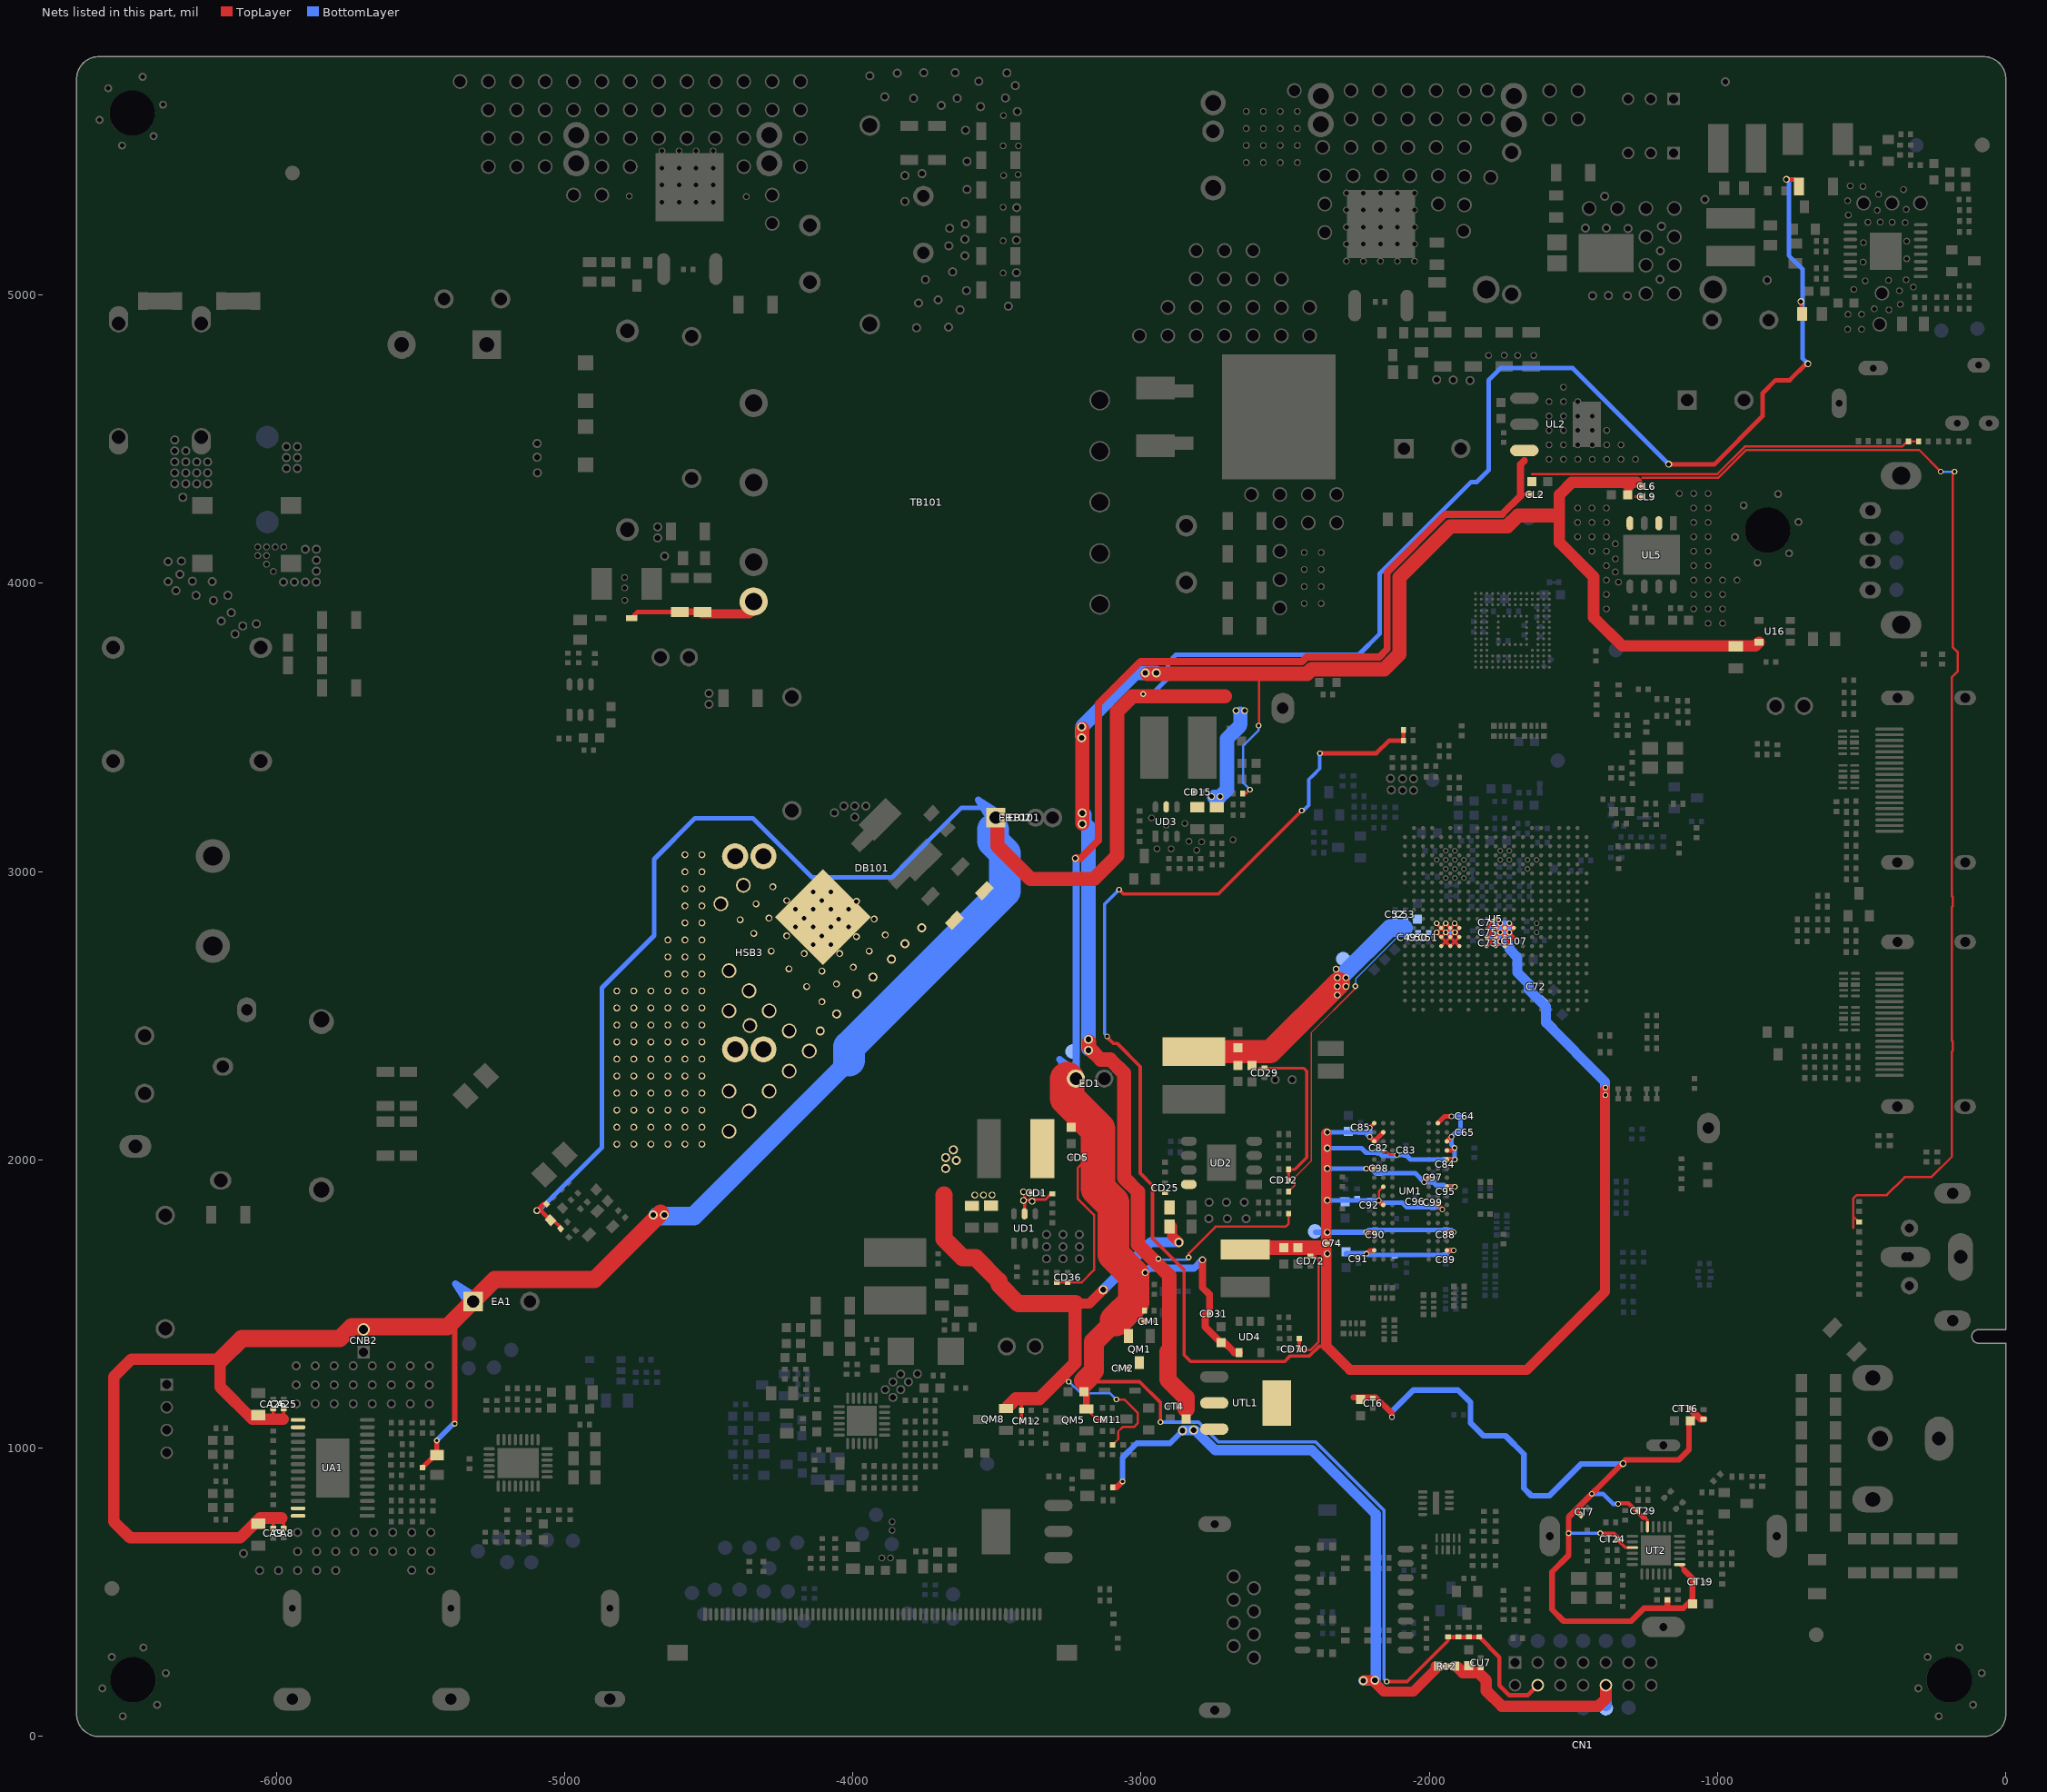
[diagram p0: the nets of this part, all layers, seen from the top]
# Altium PCB MISC84395.PcbDoc (part 9 of 26)
Units mil, origin at the board's own origin, x right, y up, seen from the top; angles counter-clockwise.
Board outline 6692.91 x 5826.77 mil, 2 copper layers (TopLayer, BottomLayer), stack 61.855 mil thick; 951 components, 565 nets, 4374 pads, 1804 vias.
Unrouted connection lines stored in the file: 1.

## Via types
v1: diameter 19.68, hole 11.81, TopLayer to BottomLayer, tented both sides, 1262 vias
v2: diameter 23.62, hole 15.75, TopLayer to BottomLayer, tented both sides, 524 vias
v3: diameter 31.5, hole 19.68, TopLayer to BottomLayer, tented both sides, 11 vias
v4: diameter 24, hole 16, TopLayer to BottomLayer, tented both sides, 6 vias
v5: diameter 19, hole 11.81, TopLayer to BottomLayer, tented both sides, 1 vias

## Nets (pads, with @x,y where several pads share a name; then routed paths per layer and width w, separated by ;. In a path a pad name is that pad's centre, name@x,y a point inside that pad or via, vN(x,y) a via of type N, cw(c..) or ccw(c..) an arc to the next point about the centre after c; other vN are vias at no path point) (continued)
3V3_TUN_IC: CT6.2 CT7.2 CT8.1 CT15.2 CT16.2 CT19.1 CT24.1 CT29.2 CT50.2 LT20.2 RT1.2 UT2.1 UT2.11 UT2.15 UTL1.2 UTL1.4 | length 3570.2
  TopLayer w10: -1334.85,670.48 -1319.68,655.32 UT2.15@-1295.78,655.32 ; -1251,758 -1243.42,750.42 UT2.11@-1243.42,727.36 ; UT2.1@-1117.02,596.26 UT2.1@-1132,596.26 -1116.5,580.76 -1116.5,577.5
  TopLayer w12: v1@-1406.82,704.82 -1358.97,704.82 -1345.48,691.34 -1345.48,680.45 -1335.39,670.35
  TopLayer w15: -1491.7,785.96 CT7.2@-1473.87,768.13 ; v1@-1343,809 -1309.42,809 -1259.97,759.55 -1251,759.55
  TopLayer w20: -2264,1176.11 -2185.43,1176.11 -2130,1120.68 ; -1174.21,447.5 RT1.2@-1174.21,474.46 ; -1116.5,577.5 -1087.44,548.44 -1087.44,476.74 ; CT8.1@-1095.5,468.68 -1118.71,445.47 -1255.17,445.47 -1300.25,400.39 -1534.23,400.39 -1574.5,440.66 -1574.5,571 -1516.97,628.53 v1(-1516.97,705) -1516.97,761.16 -1321.1,957.03 -1318.6,959.53 -1135.31,959.53 -1099.4,995.44 -1099.4,1089.79 -1098.4,1090.79 CT15.2@-1094.19,1095
  TopLayer w24: CT15.2@-1097.19,1096 CT15.2@-1096.26,1096.93 ; CT16.2@-1096.26,1137.27 -1059.26,1100.26 LT20.2@-1049,1100.26
  BottomLayer w12: v1@-1515.91,705 v1@-1408,705
  BottomLayer w15: v1(-1436.29,841.84) -1398.24,841.84 -1363.4,807 v1(-1345,807)
  BottomLayer w20: v1(-2130,1108) -2130,1127.65 -2055.8,1201.84 -1900.35,1201.84 -1857.41,1158.9 -1857.41,1088.41 -1812,1043 -1736,1043 -1672,979 -1672,860.75 -1646.25,835 -1583.89,835 -1473.59,945.3 v2@-1326.3,945.3
  other v1: -1407,705
  other v2: -1328,946.5
5V_M: CL5.2 CL6.2 CL9.2 CM2.1 CT3.2 CT4.1 CU.1 pad.VIA5@-2189,195 pad.VIA5@-2228.87,194.13 pad.VIA5@-2818,1063 pad.VIA5@-2856,1061 pad.VIA5@-2947.23,3688.77 pad.VIA5@-2985.23,3688.77 pad.VIA5@-3182.5,2380 pad.VIA5@-3182.5,2418 pad.VIA5@-3204,3165 pad.VIA5@-3204,3203 pad.VIA5@-3206,3464 pad.VIA5@-3206,3502 QM1.D R12.1 RD25.2 RD26.2 RG02.2 RI1.1 U16.5 UL5.2 UL5.4 UTL1.3 | length 13409.1
  TopLayer w8: v1(-2835,1662) -2835,1675.52 -2741.87,1768.65 -2499.35,1768.65 -2488.27,1779.73 RD25.2@-2488.27,1814 ; RD26.2@-2645.68,3269 RD26.2@-2647.56,3270.87 -2635.13,3270.87 v1(-2622,3284) ; v1@-2590.16,3508.58 -2590.16,3685.84 ; -1261,4366 -997,4366 -900.94,4462.06 -301.06,4462.06 v1(-226,4387) ; -530,1764.47 -530,1866.16 -518,1878.16 -413.16,1878.16 -351.32,1940 -258.85,1940 -187.74,2011.11 -187.74,2376.16 -184.99,2378.91 -184.99,2411.09 -187.74,2413.84 -187.74,2877.16 -184.99,2879.91 -184.99,2912.09 -187.74,2914.84 -187.74,3673.85 -167.5,3694.09 ; -530,1805 RI1.1@-509,1784 ; -184.83,3676.76 -167.5,3694.09 ; v1(-178,4387) -181,4387 -184.83,4383.17 -184.83,3779.24 -167.5,3761.91 -167.5,3694.09
  TopLayer w12: -1284.37,4336 CL6.2@-1263.11,4336 ; -1282.37,4300 CL9.2@-1263.11,4300
  TopLayer w20: RG02.2@-3098.27,864 -3085,864 v1(-3064.5,884.5)
  TopLayer w35: pad.VIA5@-2228,195 -2197.74,195 -2158.74,156 -2055.78,156 -1978.64,233.14 R12.1@-1978.64,244
  TopLayer w40: -1320.21,4350 -1308.2,4338 ; -1280.84,4350 -1506,4350 -1548.83,4307.17 -1548.83,4140.87 -1430.15,4022.18 -1430.15,3881.42 -1331.75,3783.02 -868.54,3783.02 U16.5@-855.97,3795.6
  TopLayer w50: pad.VIA5@-3203.84,3167 pad.VIA5@-3203.84,3495 ; pad.VIA5@-3180,2388 pad.VIA5@-3180,2409 ; pad.VIA5@-3177.25,2385.25 -3140.16,2348.16 -3106.98,2348.16 -3059,2300.18 -3059,1937.44 -3011,1889.44 -3011,1706.64 -2902,1597.64 -2902,1349 ; pad.VIA5@-2978,3686 -2423.73,3686 ; -2407.99,3701.75 -2423.73,3686 ; -1556.84,4235 -1691.9,4235 -1729.9,4197 -1926.83,4197 -2103.88,4019.95 -2103.88,3754.12 -2156,3702 -2407.73,3702 -2423.73,3686
  TopLayer w60: -2907,1334 -2907,1238 -2844,1175 -2844,1136
  BottomLayer w8: v1@-2939.5,1656.5 -2942,1654 -2843,1654 v1(-2835,1662) ; v1(-2622,3284) -2645.27,3307.27 -2645.27,3436.72 -2592.7,3489.29 v1(-2592.7,3506.03) ; v1(-226,4387) v1(-178,4387)
  BottomLayer w20: v1(-3064.5,884.5) -3064.29,884.71 -3064.29,967.68 -3015.16,1016.82 -2900.18,1016.82 pad.VIA5@-2856,1061
  BottomLayer w35: pad.VIA5@-2854,1062 -2812,1062 -2743.5,993.5 -2406.81,993.5 -2186,772.69 -2186,198 -2189.87,194.13 pad.VIA5@-2228.87,194.13
  BottomLayer w50: pad.VIA5@-3204,3469 -3204,3503.57 -3018.8,3688.77 pad.VIA5@-2985.23,3688.77 pad.VIA5@-2947.23,3688.77 ; pad.VIA5@-3197,3197 -3197,3169 -3182.5,3154.5 pad.VIA5@-3182.5,2418 pad.VIA5@-3182.5,2386
  other v1: -2940,1657
5V_STB: 5V_STB.1 CD5.1 CD8.2 CD31.2 CD36.2 CD69.2 CL1.2 CL2.1 CM1.1 CM3.2 CM11.2 CN1.4 ED1.1 LD1.2 QM1.S QM5.S RD1.2 RK3.2 RK5.1 RK6.2 RK12.2 RM1.2 RV15.2 RV17.2 UD4.4 UL2.3 | length 10351.8
  TopLayer w8: RD1.2@-3292,1575.54 -3205.46,1575.54 -3163,1618 -3163,1809 -3220,1866 -3220,1972 -3191,2001 ; QM5.S@-3189.76,1135.4 -3153.35,1099 CM11.2@-3133.73,1099 ; -2116.88,4072 -1975.44,4213.44 ; -1644,4378.5 -1643.5,4379 -1000.83,4379 -905.87,4473.96 -359.9,4473.96 -341.69,4492.16 RV15.2@-338.1,4492.16 -302.73,4492.16 RV17.2@-302.57,4492
  TopLayer w12: -3163.1,1230.66 -3005.44,1230.66 -2932.5,1157.72 v1(-2932.5,1090.5) ; v1(-2148,191) -2077,191 -1935,333 RK6.2@-1935,345.27 ; -1686.34,4316 -1684.33,4318 -1674.34,4308 CL2.1@-1649.73,4308
  TopLayer w15: -3025.92,1477.19 CM1.1@-2988.73,1440 ; RK6.2@-1935,345.27 RK5.1@-1861,345.27 ; RK3.2@-1889.33,345.27 RK5.1@-1861,345.27 ; RK12.2@-1824,345.27 RK12.2@-1827.21,345.27 ; CN1.4@-1624.01,178 -1659.02,143 -1723,143 -1756.91,176.91 -1756.91,274.97 RK12.2@-1827.21,345.27 ; RK5.1@-1861,345.27 RK12.2@-1827.21,345.27
  TopLayer w25: v2(-3228,3046) -3210,3046 ; v2@-3223,3046 -3210,3046 ; QM5.S@-3189.76,1135.4 -3189.76,1204 -3163.1,1230.66 ; v2(-2787.5,1653) -2787.5,1557.74 -2762.66,1532.89 -2762.66,1477.11 -2777.5,1462.26 -2777.5,1420.88 -2724.62,1368 -2712,1368 -2676.15,1332.15 UD4.4@-2659.61,1332.15 ; -2120.43,4063.5 -2146.38,4037.55 ; -1670.54,4425.45 -1684.33,4411.65 -1684.33,4318 -1684.33,4302.67 -1747.5,4239.5 -1944.43,4239.5 -2146.38,4037.55 ; -3210,3046 -3148.34,3107.66 -3148.34,3582 -3001.84,3728.5 -2441.34,3728.5 -2425.34,3744.5 -2173.6,3744.5 -2146.38,3771.72 -2146.38,4037.55
  TopLayer w70: -3198.06,1233.75 -3163.5,1268.31 -3163.5,1368.3 -3088.4,1443.4
  TopLayer w110: -3101,1852.16 -3096,1847.16 -3096,1671.43 -3025.92,1601.35 -3025.92,1505.88 -3088.4,1443.4
  TopLayer w120: ED1.1@-3256.84,2280.07 -3256.84,2213.93 -3149,2106.09 ; -3198,2156 -3149,2107 -3149,2106.09 ; -3101,1852.16 -3149,1900.16 -3149,2106.09
  BottomLayer w12: v1(-2932.5,1090.5) -2800.19,1090.5 -2731.69,1022 -2395,1022 -2157.5,784.5 -2157.5,200.5 v1(-2148,191)
  BottomLayer w25: ED1.1@-3225,2308.51 v2@-3225,3046 ; v2(-2986,1609) -2971,1624 -2816.5,1624 v2(-2787.5,1653)
5V_WIFI: 5V_WIFI.1 CN1.10 CU6.1 CU7.1 R12.2 R12.3 | length 725.1
  TopLayer w15: CN1.10@-1387.8,171.67 CN1.10@-1387.8,178
  TopLayer w40: R12.2@-1902,240 -1884,222 -1830,222 -1803,195 -1803,159 -1749,105 -1414,105 -1387.8,131.2 CN1.10@-1387.8,178
  BottomLayer w40: 5V_WIFI.1@-1387.74,108 CN1.10@-1387.74,177.95
12V: CA1.2 CA2.2 CA8.2 CA9.2 CA25.1 CA26.2 CD1.2 CD4.1 CD6.1 CD13.1 CD14.1 CD15.1 CD23.2 CD24.2 CD25.2 CM12.2 CNB2.2 DB101.2 EA1.1 EB101.1@-3504,3187 EB102.1@-3504,3187 HSB3.1 HSB3.2 HSB3.3 HSB3.4 pad.VIA5@-2641,3558 pad.VIA5@-2671,3558 pad.VIA5@-2726,3260 pad.VIA5@-2756,3260 pad.VIA5@-2869,1714 pad.VIA5@-3131.42,1549.58 pad.VIA5@-3378,1857 pad.VIA5@-3408,1859 pad.VIA5@-3408,1889 pad.VIA5@-3517,1878 pad.VIA5@-3547,1878 pad.VIA5@-3577,1878 pad.VIA5@-3641.13,1998.13 pad.VIA5@-3651,2035 pad.VIA5@-3677.87,1970.13 pad.VIA5@-3677.87,2008.13 pad.VIA5@-3761,2805 pad.VIA5@-3819,2750 pad.VIA5@-3866,2696 pad.VIA5@-3930,2634 pad.VIA5@-3986,2576 pad.VIA5@-4056,2506 pad.VIA5@-4113,2447 pad.VIA5@-4150.99,2377.82 pad.VIA5@-4220.58,2308.22 pad.VIA5@-4220.58,2447.42 pad.VIA5@-4290.18,2238.63 pad.VIA5@-4290.18,2517.02 pad.VIA5@-4357,2466 pad.VIA5@-4359.78,2169.03 pad.VIA5@-4359.78,2586.61 pad.VIA5@-4379.6,2952.4 pad.VIA5@-4429.37,2099.43 pad.VIA5@-4429.37,2238.63 pad.VIA5@-4429.38,2517.02 pad.VIA5@-4429.38,2656.21 pad.VIA5@-4457.6,2888.4 pad.VIA5@-4523.38,2054.38 pad.VIA5@-4523.38,2113.43 pad.VIA5@-4523.38,2172.49 pad.VIA5@-4523.38,2231.54 pad.VIA5@-4523.38,2290.6 pad.VIA5@-4523.38,2349.65 pad.VIA5@-4523.38,2408.71 pad.VIA5@-4523.38,2467.76 pad.VIA5@-4523.38,2526.82 pad.VIA5@-4523.38,2585.87 pad.VIA5@-4523.38,2644.93 pad.VIA5@-4523.38,2703.99 pad.VIA5@-4523.38,2763.04 pad.VIA5@-4523.38,2822.1 pad.VIA5@-4523.38,2881.15 pad.VIA5@-4523.38,2940.21 pad.VIA5@-4523.38,2999.26 pad.VIA5@-4523.38,3058.32 pad.VIA5@-4582.44,2054.38 pad.VIA5@-4582.44,2113.43 pad.VIA5@-4582.44,2172.49 pad.VIA5@-4582.44,2231.54 pad.VIA5@-4582.44,2290.6 pad.VIA5@-4582.44,2349.65 pad.VIA5@-4582.44,2408.71 pad.VIA5@-4582.44,2467.76 pad.VIA5@-4582.44,2526.82 pad.VIA5@-4582.44,2585.87 pad.VIA5@-4582.44,2644.93 pad.VIA5@-4582.44,2703.99 pad.VIA5@-4582.44,2763.04 pad.VIA5@-4582.44,2822.1 pad.VIA5@-4582.44,2881.15 pad.VIA5@-4582.44,2940.21 pad.VIA5@-4582.44,2999.26 pad.VIA5@-4582.44,3058.32 pad.VIA5@-4641.49,2054.38 pad.VIA5@-4641.49,2113.43 pad.VIA5@-4641.49,2172.49 pad.VIA5@-4641.49,2231.54 pad.VIA5@-4641.49,2290.6 pad.VIA5@-4641.49,2349.65 pad.VIA5@-4641.49,2408.71 pad.VIA5@-4641.49,2467.76 pad.VIA5@-4641.49,2526.82 pad.VIA5@-4641.49,2585.87 pad.VIA5@-4641.49,2644.93 pad.VIA5@-4641.49,2703.99 pad.VIA5@-4641.49,2763.04 pad.VIA5@-4654,1809 pad.VIA5@-4692,1809 pad.VIA5@-4700.55,2054.38 pad.VIA5@-4700.55,2113.43 pad.VIA5@-4700.55,2172.49 pad.VIA5@-4700.55,2231.54 pad.VIA5@-4700.55,2290.6 pad.VIA5@-4700.55,2349.65 pad.VIA5@-4700.55,2408.71 pad.VIA5@-4700.55,2467.76 pad.VIA5@-4700.55,2526.82 pad.VIA5@-4700.55,2585.87 pad.VIA5@-4759.6,2054.38 pad.VIA5@-4759.6,2113.43 pad.VIA5@-4759.6,2172.49 pad.VIA5@-4759.6,2231.54 pad.VIA5@-4759.6,2290.6 pad.VIA5@-4759.6,2349.65 pad.VIA5@-4759.6,2408.71 pad.VIA5@-4759.6,2467.76 pad.VIA5@-4759.6,2526.82 pad.VIA5@-4759.6,2585.87 pad.VIA5@-4818.66,2054.38 pad.VIA5@-4818.66,2113.43 pad.VIA5@-4818.66,2172.49 pad.VIA5@-4818.66,2231.54 pad.VIA5@-4818.66,2290.6 pad.VIA5@-4818.66,2349.65 pad.VIA5@-4818.66,2408.71 pad.VIA5@-4818.66,2467.76 pad.VIA5@-4818.66,2526.82 pad.VIA5@-4818.66,2585.87 QM8.S R27.2 RA25.1 RA27.1 RB128.2 RB129.2 RB131.2 RB135.1 RB158.2 RB816.2 RB826.2 RD2.1 RM2.1 UA1.15 UA1.16 UA1.27 UA1.28 UD1.5 UD2.8 UD3.5 | length 17762
  TopLayer w8: -3271.72,1251.72 v1(-3251,1231) ; R27.2@-3099,1011.73 -3079.41,1031.32 -3079.41,1058.09 -3063.75,1073.75 -3024.41,1073.75 -3012,1086.16 -3012,1123 -3058,1169 v1(-3086,1169)
  TopLayer w10: UD1.5@-3404,1813.18 pad.VIA5@-3404,1861 ; -3404,1871.89 pad.VIA5@-3404,1861 ; pad.VIA5@-3383.84,1862.16 -3332.18,1862.16 -3312.61,1881.73 RD2.1@-3308,1881.73 ; pad.VIA5@-3378,1861 pad.VIA5@-3404,1861
  TopLayer w11.81: v2(-711,4977) -711,4938.41 RB816.2@-706.59,4934
  TopLayer w12: -6010.52,1102.69 CA26.2@-6010.52,1136.51 ; CA9.2@-6010.23,722 -6010.23,753.66 ; CA8.2@-5974.23,722.26 -5974.23,751 ; -5974.18,1101.86 CA25.1@-5974.18,1136.5 ; RA25.1@-5492.6,932.67 RA25.1@-5485.96,932.67 ; RB131.2@-5038.61,1790.94 RB135.1@-5010.83,1763.17 ; CM12.2@-3414.74,1095 -3414.74,1151.89
  TopLayer w15: RB826.2@-718.06,5376 RB826.2@-717.06,5375
  TopLayer w15.75: RB158.2@-5062.78,1846.33 -5073.67,1846.33 v2(-5096,1824) -5082.11,1824 RB131.2@-5049.06,1790.94 ; v2(-1170,4413) -1010.63,4413 -843.74,4579.89 -843.74,4659.39 -799,4704.13 -749.89,4704.13 -693.02,4761 v2(-687,4761) ; v2(-762,5401) -734,5401 -718.06,5385.06 RB826.2@-718.06,5376
  TopLayer w18: RA25.1@-5492.6,932.67 RA27.1@-5445.91,979.35 ; v1@-5443.07,1024.6 -5443.07,976.51 RA27.1@-5442.6,976.03 ; v1(-5380.94,1085) -5380.94,1414
  TopLayer w35: -3229,1501.5 -3179.5,1501.5 pad.VIA5@-3131.42,1549.58 ; CD23.2@-2892,1769 -2892,1737 pad.VIA5@-2869,1714
  TopLayer w40: -5981.23,758 -6056.3,758 -6125.08,689.21 -6506.95,689.21 -6564,746.26 -6564,1247.13 -6502,1309.13 -6194.94,1309.13 -6194.94,1212.73 -6082.61,1100.4 -5975.63,1100.4
  TopLayer w45: QM8.S@-3461.58,1144.58 -3434.5,1171.66 -3352.78,1171.66 -3229,1295.44 -3229,1501.5
  TopLayer w50: EB102.1@-3498.52,3187 -3498.52,3089.52 -3383.5,2974.5 -3163.86,2974.5 -3082.84,3055.52 -3082.84,3554.87 -3029.71,3608 -2710.12,3608
  TopLayer w60: -6191.08,1309.13 -6120.02,1380.19 -5779.76,1380.19 -5737.94,1422 -5421.49,1422 -5405.43,1422 -5242.58,1584.85 -4896.22,1584.85 pad.VIA5@-4666.54,1814.54 ; -3683.73,1878 -3683.73,1726.07 -3618.41,1660.75 -3574.14,1660.75 -3493.39,1580.01 -3493.39,1569.43 -3425.47,1501.5 -3229,1501.5
  BottomLayer w8: v1(-3251,1231) -3250,1231 -3209.84,1190.84 -3107.84,1190.84 v1(-3086,1169)
  BottomLayer w15.75: v2@-5092.5,1820.5 -4870.25,2042.75 -4870.25,2597.16 -4689.25,2778.16 -4689.25,3043.16 -4547.16,3185.25 -4346.84,3185.25 -4140.84,2979.25 -3865.16,2979.25 -3622.72,3221.69 ; -3548.65,3221.69 -3622.72,3221.69 ; EB102.1@-3504,3187 -3538.69,3221.69 -3622.72,3221.69 ; v1(-2993,3616) -2962.2,3616 -2906.35,3671.84 -2906.35,3724.65 -2879.24,3751.76 -2245.12,3751.76 -2171.76,3825.12 -2171.76,4034.24 -1854.5,4351.5 -1835.5,4351.5 -1795,4392 -1795,4704 -1753,4746 -1503,4746 v2(-1170,4413) ; v2(-762,5401) -753,5392 -753,5136.83 -706,5089.83 -706,4780 v2(-687,4761)
  BottomLayer w18: v1@-5442.92,1027.51 v1@-5385.42,1085
  BottomLayer w35: pad.VIA5@-3131.42,1549.58 -2967,1714 pad.VIA5@-2869,1714
  BottomLayer w50: pad.VIA5@-2746,3258.16 -2745.53,3258.63 -2727.37,3258.63 -2702.27,3283.73 -2702.27,3460.33 -2657.16,3505.44 -2657.16,3510.39 -2655.55,3512 -2655.55,3548
  BottomLayer w65: -4676.37,1805.63 -4551.48,1805.63 -4012.43,2344.68 -4012.43,2369.43
  BottomLayer w110: -4012.43,2344.68 -4012.43,2392.34 -3473,2931.77 -3473,3064 -3514,3105 -3514,3146
  other v1: -5442.92,1026.51
  other v2: -4107.18,2548.72 -4160.07,2601.61 -4057.07,2609.96 -4107.18,2654.5 -4221.32,2662.86 -3998.61,2668.42 -4168.43,2715.75 -4045.94,2715.75 -4282.57,2724.1 -3942.93,2724.1 -4137.8,2746.37 -4076.56,2746.37 -3987.47,2774.21 -4229.67,2777 -4107.18,2777 -3887.25,2779.78 -4343.81,2785.35 -4199.05,2807.62 -4137.8,2807.62 -4076.56,2807.62 -4015.31,2807.62 -4391.14,2832.67 -4048.72,2835.46 -3926.23,2835.46 -4290.92,2838.24 -4168.43,2838.24 -4199.05,2868.86 -4137.8,2868.86 -4076.56,2868.86 -4015.31,2868.86 -4335.46,2888.35 -3987.47,2896.7 -4229.67,2899.49 -4107.18,2899.49 -4137.8,2930.11 -4076.56,2930.11 -4277,2946.81
12V_OVP: DB121.A RB114.2 RB115.2 TB101.6@-4344.32,3936.02 | length 442.8
  TopLayer w15.75: DB121.A@-4767.85,3879 -4746.55,3900.3 RB114.2@-4600,3900.3
  TopLayer w23.62: RB114.2@-4604,3900.19 -4523.24,3900.19 RB115.2@-4523.16,3900.11
  TopLayer w31.5: RB115.2@-4523.24,3893.11 -4359.67,3893.11 TB101.6@-4344.32,3908.46
+1.5V_DDR: +1.5V_DDR.1 C64.1 C65.2 C71.2 C72.2 C73.2 C74.2 C75.2 C80.2 C81.2 C82.2 C83.2 C84.2 C85.2 C87.2 C88.2 C89.2 C90.2 C91.2 C92.2 C94.2 C95.2 C96.2 C97.2 C98.2 C99.2 C104.2 C105.2 C106.2 C107.2 CD70.2 CD72.2 CD73.1 CD74.1 LD5.2 pad.VIA5@-1389.65,2224.74 pad.VIA5@-1389.65,2250.74 pad.VIA5@-1722.72,2788.84 pad.VIA5@-1722.72,2820.34 pad.VIA5@-1754.22,2757.34 pad.VIA5@-1754.22,2788.84 pad.VIA5@-1754.22,2820.34 R46.2 R48.1 R51.2 RD50.2 RM10.2 U5.H10 U5.H11 U5.H12 U5.J10 U5.J11 U5.J12 U5.K9 U5.K10 U5.K11 U5.L11 UM1.A1 UM1.A8 UM1.B2 UM1.C1 UM1.C9 UM1.D2 UM1.D9 UM1.E9 UM1.F1 UM1.G7 UM1.H2 UM1.H9 UM1.K2 UM1.K8 UM1.N1 UM1.N9 UM1.R1 UM1.R9 | length 11795.6
  TopLayer w7.87: v1(-2175.48,1859.7) -2175.48,1891.2 UM1.H2@-2159.73,1906.95 ; UM1.D2@-2159.73,2032.93 -2159.73,2028.99 -2147.92,2028.99 -2136.11,2017.18 v1(-2112.49,2017.18)
  TopLayer w8: CD70.2@-2447.74,1340 -2414,1340 -2384,1370 -2384,1653 -2396.83,1665.83 CD72.2@-2413,1665.83
  TopLayer w10: U5.H12@-1801.46,2741.6 -1785.72,2757.34 ; -1785.72,2757.34 U5.J11@-1769.97,2773.09 ; -1785.72,2757.34 U5.H11@-1769.97,2741.6 pad.VIA5@-1754.22,2757.34 ; -1785.72,2757.34 U5.J12@-1801.46,2773.09 -1785.72,2788.84 ; -1785.72,2788.84 -1801.46,2804.59 -1785.72,2820.34 ; -1785.72,2788.84 U5.J11@-1769.97,2773.09 ; -1785.72,2788.84 U5.K11@-1769.97,2804.59 ; -1785.72,2820.34 U5.L11@-1769.97,2836.08 pad.VIA5@-1754.22,2820.34 ; -1785.72,2820.34 U5.K11@-1769.97,2804.59 ; U5.J11@-1769.97,2773.09 pad.VIA5@-1754.22,2788.84 ; U5.J11@-1769.97,2773.09 pad.VIA5@-1754.22,2757.34 ; U5.K11@-1769.97,2804.59 pad.VIA5@-1754.22,2788.84 ; U5.K11@-1769.97,2804.59 pad.VIA5@-1754.22,2820.34 ; pad.VIA5@-1754.22,2757.34 U5.J10@-1738.47,2773.09 ; pad.VIA5@-1754.22,2757.34 U5.H10@-1738.47,2741.6 -1722.72,2757.34 ; pad.VIA5@-1754.22,2788.84 U5.J10@-1738.47,2773.09 ; pad.VIA5@-1754.22,2788.84 U5.K10@-1738.47,2804.59 ; pad.VIA5@-1754.22,2820.34 U5.K10@-1738.47,2804.59 ; U5.J10@-1738.47,2773.09 pad.VIA5@-1722.72,2788.84 ; U5.J10@-1738.47,2773.09 -1722.72,2757.34 ; U5.K10@-1738.47,2804.59 pad.VIA5@-1722.72,2820.34 U5.K9@-1706.98,2804.59 pad.VIA5@-1722.72,2788.84 ; U5.K10@-1738.47,2804.59 pad.VIA5@-1722.72,2788.84 ; -1722.72,2757.34 -1706.98,2773.09 pad.VIA5@-1722.72,2788.84
  TopLayer w12: v1@-3118,2425.52 -3096.63,2404.16 -3083.78,2404.16 -3003,2323.38 -3003,1953.57 -2960,1910.57 -2960,1727.77 -2851,1618.77 -2851,1324 -2828,1301 -2502.09,1301 -2483.09,1320 -2416,1320 -2382.33,1353.67 -2357.57,1353.67 ; v1@-3071.5,2932.5 -3061.5,2922.5 -2731.45,2922.5 v1(-2442.47,3211.48) ; CD70.2@-2451.27,1343.53 RD50.2@-2451.27,1380.26 ; v1(-2206.98,2111.67) UM1.A1@-2191.23,2127.42
  TopLayer w15: v1(-2380,3410.34) -2183.66,3410.34 -2140,3454 R46.2@-2089.73,3454 R48.1@-2089.73,3491 ; v1(-2218.79,1969.94) UM1.F1@-2191.23,1969.94
  TopLayer w15.75: v1(-2218.79,1749.47) UM1.N1@-2191.23,1749.47 ; v1(-2217.8,1674.66) -2205.99,1686.47 UM1.R1@-2191.23,1686.48 ; v1(-2206.98,2080.17) UM1.C1@-2191.23,2064.43 UM1.B2@-2159.73,2095.93 ; v1(-2175.48,1859.7) UM1.K2@-2159.73,1843.96 ; v1(-2018,1922.7) UM1.G7@-2002.25,1938.45 ; UM1.K8@-1970.75,1843.96 v1(-1955.01,1828.21) ; UM1.A8@-1970.75,2127.42 -1947.13,2151.04 v1(-1923.51,2151.04) ; UM1.R9@-1939.26,1686.48 v1(-1915.64,1686.48) ; UM1.N9@-1939.26,1749.47 v1(-1915.64,1749.47) ; UM1.H9@-1939.26,1906.95 v1(-1911.7,1906.95) ; UM1.E9@-1939.26,2001.44 v1(-1911.7,2001.43) ; UM1.D9@-1939.26,2032.93 -1921.54,2032.93 v1(-1912.69,2041.79) ; UM1.C9@-1939.26,2064.43 v1(-1923.51,2080.17)
  TopLayer w35: v4@-2357.57,2092.48 -2357.57,1353.67 -2275.52,1271.61 -1662.22,1271.61 -1390.67,1543.16 pad.VIA5@-1390.67,2244
  TopLayer w50: LD5.2@-2639,1689.22 -2633.15,1695.07 CD74.1@-2505,1695.07 CD73.1@-2456,1695.07 -2365.44,1695.07
  BottomLayer w12: -3126.5,2437.5 -3126.5,2886.5 v1(-3076,2937) ; v1(-2442.47,3211.48) -2437.52,3211.48 -2418.25,3230.75 -2418.25,3319.25 -2404.48,3333.02 -2404.29,3333.02 -2380,3357.3 v1(-2380,3410.34)
  BottomLayer w15.75: v4(-2353.97,1859.7) v1(-2175.48,1859.7) -2167.61,1851.83 -2094.31,1851.83 -2078.25,1835.77 -1962.57,1835.77 ; v4(-2353.97,1969.94) v1(-2218.79,1969.94) -2203.36,1969.94 -2187.29,1953.88 -2049.18,1953.88 v1(-2018,1922.7) C97.2@-1986.51,1922.69 ; v4(-2353.97,2040.8) -2235.72,2040.8 -2219.97,2025.06 C82.2@-2175.48,2025.06 -2164.66,2014.23 -2115.44,2014.23 v1(-2112.49,2017.18) C83.2@-2080.99,2017.18 -2065.25,2001.43 v1(-1911.7,2001.43) -1911.7,2040.8 v1(-1912.69,2041.79) -1923.51,2052.62 v1(-1923.51,2080.17) -1909.73,2093.95 -1892.33,2093.95 -1892.33,2151.04 C64.1@-1892.99,2151.08 v1(-1923.51,2151.04) ; v4(-2353.97,2096.08) C85.2@-2238.47,2096.08 -2238.47,2095.92 -2222.73,2095.92 ; v1(-2218.79,1749.47) -2210.61,1757.65 -1923.51,1757.65 ; v1@-2214.18,1671.04 C89.2@-1943.2,1671.05 -1927.77,1686.48 v1(-1915.64,1686.48) ; v1(-2206.98,2080.17) -2222.73,2095.92 ; v1(-2206.98,2111.67) -2222.73,2095.92 ; v1(-1911.7,1906.95) C95.2@-1943.2,1906.96 ; C97.2@-1986.51,1922.69 -1970.77,1906.95 C95.2@-1943.2,1906.96 ; C97.2@-1986.51,1922.69 -1976.66,1912.85 -1949.1,1912.85 C95.2@-1943.2,1906.96
  BottomLayer w19.68: +1.5V_DDR.1@-2394.47,1749.47 v1(-2218.79,1749.47) ; C87.2@-2288.48,1674.66 v1(-2217.8,1674.66) ; -1781.78,2800.65 -1781.65,2800.5 -1779,2797.32 -1778.61,2796.85 -1777.49,2795.5 C75.2@-1774.67,2792.11 ; C75.2@-1774.66,2792.11 C75.2@-1771.94,2788.84
  BottomLayer w19.69: v1(-2206.98,2080.17) v1(-2206.98,2111.67)
  BottomLayer w20: C73.2@-1781.78,2753.41 -1736.5,2753.41 -1726.66,2753.41 -1722.72,2757.34 pad.VIA5@-1722.72,2788.84 pad.VIA5@-1722.72,2820.34 ; C75.2@-1781.78,2796.08 -1781.78,2800.65 ; pad.VIA5@-1754.22,2820.34 pad.VIA5@-1722.72,2820.34 ; pad.VIA5@-1722.35,2820.34 pad.VIA5@-1722.72,2820.34
  BottomLayer w24: C73.2@-1781.78,2753.41 C75.2@-1781.78,2796.08 ; -1781.78,2800.65 -1781.62,2800.81 -1773.97,2808.46 -1741.97,2808.46 -1741.97,2773.48 ; -1756.57,2773.48 -1741.97,2773.48 ; -1724.57,2773.48 -1741.97,2773.48
  BottomLayer w35: C75.2@-1771.94,2788.84 -1756.57,2773.48 -1747.33,2764.23 -1736.5,2753.41 -1733.71,2750.61 -1731.44,2748.34 -1730.57,2747.48 -1722.2,2739.1 -1722.2,2730.31 -1695.16,2703.28 -1695.16,2651.16 -1655.24,2611.23 -1655.24,2590.9 -1595.83,2531.5 -1595.83,2476.39 -1390.68,2271.23 pad.VIA5@-1390.68,2230.74
  other v1: -3118,2428
  other v4: -2353.97,1674.67 -2353.97,1748.49
+1.05V_VDDC_CPU: +1.05V_VDDC_CPU.1 C45.2 C46.2 C47.2 C48.2 C49.2 C50.2 C51.2 C52.2 C53.2 CD2.2 CD12.2 CD26.2 CD28.2 CD29.1 LD2.2 pad.VIA5@-1911.7,2788.84 pad.VIA5@-1912.18,2820.33 pad.VIA5@-1943.2,2788.84 pad.VIA5@-1943.2,2820.34 pad.VIA5@-1974.69,2788.84 pad.VIA5@-1974.69,2820.34 pad.VIA5@-2289.65,2601.74 pad.VIA5@-2289.65,2631.74 pad.VIA5@-2319.65,2571.74 pad.VIA5@-2319.65,2601.74 pad.VIA5@-2319.65,2631.74 pad.VIA5@-2323.65,2661.74 RD7.2 RD12.2 U5.H15 U5.H16 U5.H17 U5.J15 U5.J16 U5.J17 U5.K15 U5.K16 U5.K17 | length 3056.2
  TopLayer w5: RD12.2@-2488.27,1890 -2466,1912.27 -2466,1940 -2410.07,1995.93 -2410.07,2440.93 v1@-2256.65,2594.35
  TopLayer w10: -2590.02,2317.75 -2435.32,2317.75 -2425.57,2308 -2425.57,2008.08 -2466.65,1967 RD7.2@-2488.27,1967 CD12.2@-2488.27,1929 ; CD29.1@-2572,2318.73 CD29.1@-2571.02,2317.75 ; pad.VIA5@-1974.69,2820.34 U5.K17@-1958.94,2804.59 ; U5.H17@-1958.94,2741.6 -1943.2,2757.34 ; pad.VIA5@-1912.18,2820.33 pad.VIA5@-1911.38,2820.33 ; U5.H15@-1895.95,2741.6 -1911.7,2757.34 ; U5.J17@-1958.94,2773.09 pad.VIA5@-1943.2,2788.84 ; U5.J17@-1958.94,2773.09 pad.VIA5@-1974.69,2788.84 U5.K17@-1958.94,2804.59 ; U5.J17@-1958.94,2773.09 -1943.2,2757.34 ; U5.K17@-1958.94,2804.59 pad.VIA5@-1943.2,2820.34 U5.K16@-1927.45,2804.59 ; U5.K17@-1958.94,2804.59 pad.VIA5@-1943.2,2788.84 ; -1943.2,2757.34 U5.H16@-1927.45,2741.6 -1911.7,2757.34 ; -1943.2,2757.34 U5.J16@-1927.45,2773.09 ; pad.VIA5@-1943.2,2788.84 U5.J16@-1927.45,2773.09 ; pad.VIA5@-1943.2,2788.84 U5.K16@-1927.45,2804.59 ; U5.J16@-1927.45,2773.09 pad.VIA5@-1911.7,2788.84 ; U5.J16@-1927.45,2773.09 -1911.7,2757.34 ; U5.K16@-1927.45,2804.59 -1927.12,2804.59 pad.VIA5@-1911.38,2820.33 ; U5.K16@-1927.45,2804.59 pad.VIA5@-1911.7,2788.84 ; -1911.7,2757.34 U5.J15@-1895.95,2773.09 pad.VIA5@-1911.7,2788.84 ; pad.VIA5@-1911.7,2788.84 U5.K15@-1895.95,2804.59 -1895.95,2804.91 pad.VIA5@-1911.38,2820.33
  TopLayer w80: LD2.2@-2799,2375.87 -2551.51,2375.87 -2314.65,2612.74
  BottomLayer w5: v1(-2256.65,2602.74) -2255.65,2603.74 -2255.65,2628.08 -2100.82,2782.91 ; -2087.2,2788.45 C49.2@-2076.48,2788.46
  BottomLayer w19.68: pad.VIA5@-1943.2,2788.84 pad.VIA5@-1911.7,2788.84
  BottomLayer w60: -2303.65,2636.74 -2136.26,2804.12 -2087.15,2804.12